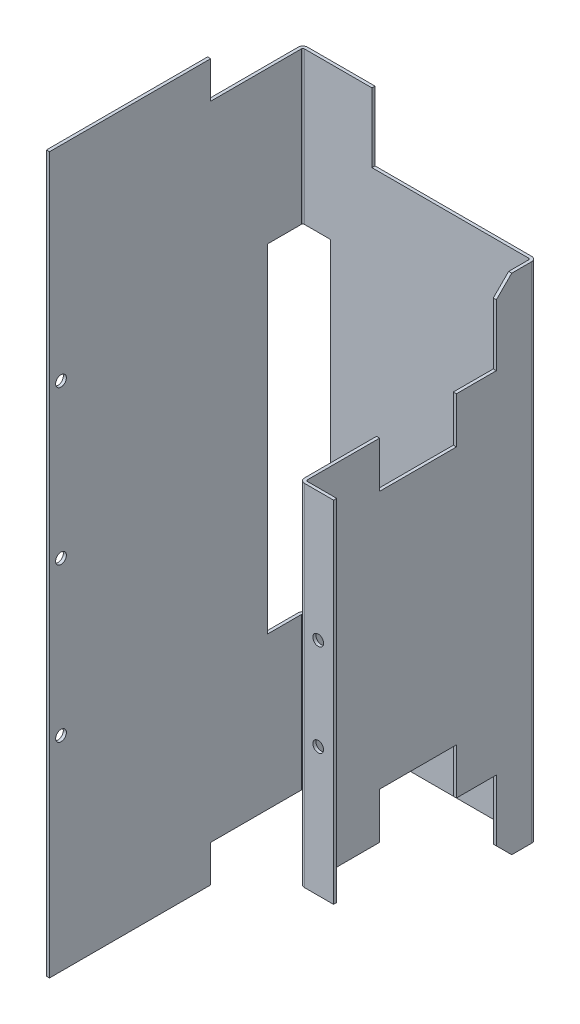
from build123d import *

# Parameters (mm, degrees)
BOSS_EXTRUDE1_DEPTH     = 418
SKETCH2_W               = 20
SKETCH2_H               = 220
CUT_EXTRUDE1_DEPTH      = 25
SKETCH3_W               = 125
SKETCH3_H               = 45
CUT_EXTRUDE2_DEPTH      = 482.157978215
FILLET1_R               = 3
FILLET2_R               = 1
SKETCH5_R               = 3.5
CUT_EXTRUDE4_DEPTH      = 476.524973056
CUT_EXTRUDE5_REACH      = 483.868
SKETCH6_R               = 3.5
SKETCH8_W               = 2
SKETCH8_H               = 105
BOSS_EXTRUDE2_DEPTH     = 24
SKETCH9_W               = 2
SKETCH9_H               = 105
BOSS_EXTRUDE3_DEPTH     = 24
CUT_EXTRUDE6_DEPTH      = 30
CUT_EXTRUDE6_DEPTH_BACK = 10
SKETCH10_W              = 126
SKETCH10_H              = 50
CHAMFER1_SIZE           = 10
SKETCH11_W              = 50
SKETCH11_H              = 30
CUT_EXTRUDE7_DEPTH      = 10


with BuildPart() as part:
    # Sketch1 → Boss-Extrude1 (new body)
    with BuildSketch(Plane(origin=(0, 0, 0), x_dir=(1, 0, 0), z_dir=(0, 1, 0))):
        Polygon((0, 0), (0, 165), (148, 165), (148, 15), (170, 15), (170, 17), (150, 17), (150, 167), (-2, 167), (-2, 0), align=None)
    extrude(amount=BOSS_EXTRUDE1_DEPTH)

    # Sketch2 → Cut-Extrude1 (cut)
    with BuildSketch(Plane(origin=(0, 0, -167), x_dir=(-1, 0, 0), z_dir=(0, 0, -1))):
        with Locations((-8, 209)):
            Rectangle(SKETCH2_W, SKETCH2_H)
    extrude(amount=-CUT_EXTRUDE1_DEPTH, mode=Mode.SUBTRACT)

    # Sketch3 → Cut-Extrude2 (cut, through all)
    with BuildSketch(Plane(origin=(0, 0, -167), x_dir=(-1, 0, 0), z_dir=(0, 0, -1))):
        with Locations((-107.5, 395.5)):
            Rectangle(SKETCH3_W, SKETCH3_H)
        with Locations((-107.5, 22.5)):
            Rectangle(SKETCH3_W, SKETCH3_H)
    extrude(amount=-CUT_EXTRUDE2_DEPTH, mode=Mode.SUBTRACT)

    # Fillet1
    fillet1_edges = [part.edges().sort_by_distance(p)[0] for p in [
        (-2, 368.5, -167),
        (-2, 49.5, -167),
        (150, 209, -167),
        (148, 209, -15),
    ]]
    fillet(fillet1_edges, radius=FILLET1_R)

    # Fillet2
    fillet2_edges = [part.edges().sort_by_distance(p)[0] for p in [
        (0, 368.5, -165),
        (0, 49.5, -165),
        (150, 209, -17),
        (148, 209, -165),
    ]]
    fillet(fillet2_edges, radius=FILLET2_R)

    # Sketch5 → Cut-Extrude4 (cut, through all)
    with BuildSketch(Plane(origin=(0, 0, -17), x_dir=(-1, 0, 0), z_dir=(0, 0, -1))):
        with Locations((-160, 239)):
            Circle(SKETCH5_R)
        with Locations((-160, 179)):
            Circle(SKETCH5_R)
    extrude(amount=-CUT_EXTRUDE4_DEPTH, mode=Mode.SUBTRACT)

    # Sketch6 → Cut-Extrude5 (cut, up to next)
    with BuildSketch(Plane.ZY.offset(2), mode=Mode.PRIVATE) as cut_extrude5_sk1:
        with Locations((-7.5, 309)):
            Circle(SKETCH6_R)
    cut_extrude5_tool1 = extrude(cut_extrude5_sk1.sketch, amount=-CUT_EXTRUDE5_REACH, mode=Mode.PRIVATE) & part.part
    # Sketch6 → Cut-Extrude5 (cut, up to next)
    with BuildSketch(Plane.ZY.offset(2), mode=Mode.PRIVATE) as cut_extrude5_sk2:
        with Locations((-7.5, 209)):
            Circle(SKETCH6_R)
    cut_extrude5_tool2 = extrude(cut_extrude5_sk2.sketch, amount=-CUT_EXTRUDE5_REACH, mode=Mode.PRIVATE) & part.part
    # Sketch6 → Cut-Extrude5 (cut, up to next)
    with BuildSketch(Plane.ZY.offset(2), mode=Mode.PRIVATE) as cut_extrude5_sk3:
        with Locations((-7.5, 109)):
            Circle(SKETCH6_R)
    cut_extrude5_tool3 = extrude(cut_extrude5_sk3.sketch, amount=-CUT_EXTRUDE5_REACH, mode=Mode.PRIVATE) & part.part
    add(cut_extrude5_tool1.solids().sort_by_distance((-2, 309, -7.5))[0], mode=Mode.SUBTRACT)
    add(cut_extrude5_tool2.solids().sort_by_distance((-2, 209, -7.5))[0], mode=Mode.SUBTRACT)
    add(cut_extrude5_tool3.solids().sort_by_distance((-2, 109, -7.5))[0], mode=Mode.SUBTRACT)

    # Sketch8 → Boss-Extrude2 (add)
    with BuildSketch(Plane.XZ):
        with Locations((-1, -52.5)):
            Rectangle(SKETCH8_W, SKETCH8_H)
    extrude(amount=BOSS_EXTRUDE2_DEPTH)

    # Sketch9 → Boss-Extrude3 (add)
    with BuildSketch(Plane(origin=(0, 418, 0), x_dir=(1, 0, 0), z_dir=(0, 1, 0))):
        with Locations((-1, 52.5)):
            Rectangle(SKETCH9_W, SKETCH9_H)
    extrude(amount=BOSS_EXTRUDE3_DEPTH)

    # Sketch10 → Cut-Extrude6 (cut, two sides: drawn at the far end of the back side and taken through both)
    with BuildSketch(Plane(origin=(150, 0, 0), x_dir=(0, 0, -1), z_dir=(1, 0, 0)).offset(-CUT_EXTRUDE6_DEPTH_BACK)):
        with Locations((78, 348)):
            Rectangle(SKETCH10_W, SKETCH10_H)
        with Locations((78, 70)):
            Rectangle(SKETCH10_W, SKETCH10_H)
    extrude(amount=CUT_EXTRUDE6_DEPTH + CUT_EXTRUDE6_DEPTH_BACK, mode=Mode.SUBTRACT)

    # Chamfer1
    chamfer1_edges = [part.edges().sort_by_distance(p)[0] for p in [
        (149, 373, -141),
        (149, 45, -141),
    ]]
    chamfer(chamfer1_edges, length=CHAMFER1_SIZE)

    # Sketch11 → Cut-Extrude7 (cut)
    with BuildSketch(Plane(origin=(150, 0, 0), x_dir=(0, 0, -1), z_dir=(1, 0, 0))):
        with Locations((90, 110)):
            Rectangle(SKETCH11_W, SKETCH11_H)
        with Locations((90, 308)):
            Rectangle(SKETCH11_W, SKETCH11_H)
    extrude(amount=-CUT_EXTRUDE7_DEPTH, mode=Mode.SUBTRACT)


solid = part.part
